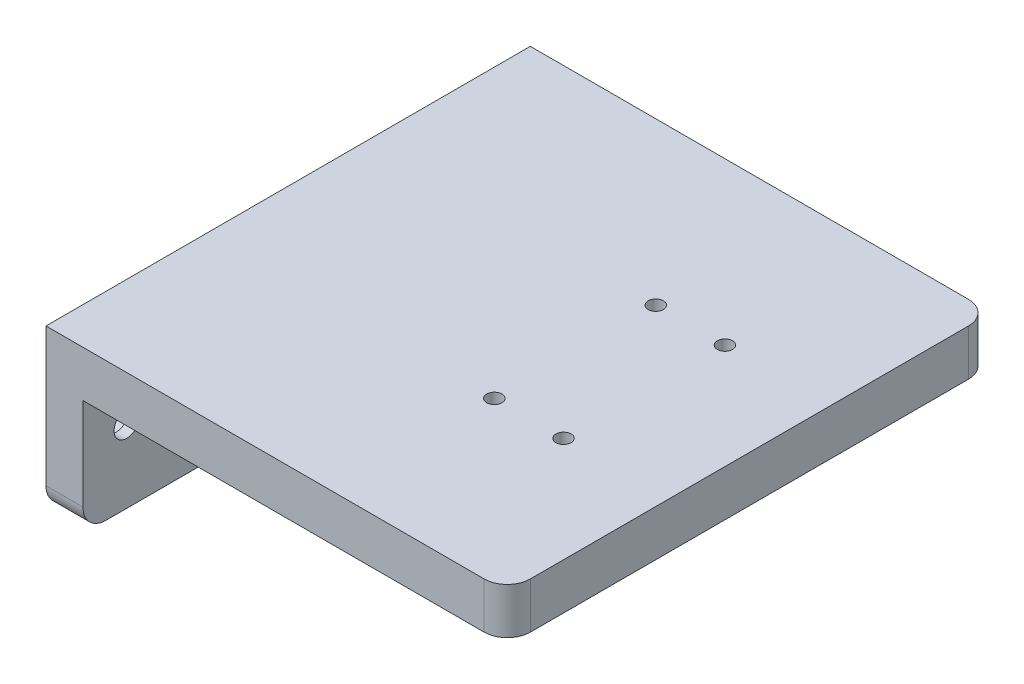
from build123d import *

# Parameters (mm, degrees)
EXTRUDE_1_DEPTH              = 27
SKETCH_2_R                   = 16
CUT_EXTRUDE_1_DEPTH          = 107.437775249
EXTRUDE_START                = -1.2
SKETCH_3_R                   = 16
SKETCH_3_R_2                 = 15
EXTRUDE_1_2_DEPTH            = 1.2
SKETCH_5_W                   = 100
SKETCH_5_H                   = 105
EXTRUDE_2_DEPTH              = 10
FILLET_1_R                   = 5
HOLE_WIZARD_M4_1_D           = 3.3
SKETCH_10_W                  = 21.869488537
SKETCH_10_H                  = 58.553791887
CUT_EXTRUDE_2_DEPTH          = 50
SKETCH_11_W                  = 105
SKETCH_11_H                  = 35
EXTRUDE_3_DEPTH              = 8
HOLE_WIZARD_M5_1_D           = 5.5
HOLE_WIZARD_M5_1_DEPTH       = 10.1
HOLE_WIZARD_M5_1_CBORE_D     = 10
HOLE_WIZARD_M5_1_CBORE_DEPTH = 5.7
HOLE_WIZARD_M5_1_TIP         = 1.652366702
FILLET_2_R                   = 5


with BuildPart() as part:
    # 草图1 → Extrude 1 (new, symmetric)
    with BuildSketch(Plane.XY):
        Polygon((90, 0), (0, 0), (0, 50), (-10, 50), (-10, -10), (90, -10), align=None)
    extrude(amount=EXTRUDE_1_DEPTH, both=True)

    # 草图2 → 切除-拉伸1 (cut, through all)
    with BuildSketch(Plane(origin=(0, 0, 0), x_dir=(0, 0, -1), z_dir=(1, 0, 0))):
        with Locations((0, 30)):
            Circle(SKETCH_2_R)
    extrude(amount=-CUT_EXTRUDE_1_DEPTH, mode=Mode.SUBTRACT)

    # 草图3 → Extrude 1 2 (add)
    with BuildSketch(Plane.ZY.offset(10).offset(EXTRUDE_START)):
        with Locations(Location((0, 30, 0), (0, 0, 180))):
            Circle(SKETCH_3_R)
        with Locations((0, 30)):
            Circle(SKETCH_3_R_2, mode=Mode.SUBTRACT)
    extrude(amount=EXTRUDE_1_2_DEPTH)

    # 草图5 → 凸台-拉伸2 (add)
    with BuildSketch(Plane(origin=(0, 0, 0), x_dir=(1, 0, 0), z_dir=(0, 1, 0))):
        with Locations((40, 0)):
            Rectangle(SKETCH_5_W, SKETCH_5_H)
    extrude(amount=-EXTRUDE_2_DEPTH)

    # 圆角1
    fillet_1_edges = [part.edges().sort_by_distance(p)[0] for p in [
        (-5, 50, 27),
        (90, -5, -52.5),
        (90, -5, 52.5),
        (-5, 50, -27),
    ]]
    fillet(fillet_1_edges, radius=FILLET_1_R)

    # M4 螺纹孔1 (through all)
    with Locations(Plane(origin=(67.2, 0, 17.5), x_dir=(0, 0, 1), z_dir=(0, 1, 0))):
        with Locations((0, 0), (0, -15), (-35, 0), (-35, -15)):
            Hole(HOLE_WIZARD_M4_1_D / 2)

    # 草图10 → 切除-拉伸2 (cut)
    with BuildSketch(Plane(origin=(0, 50, 0), x_dir=(1, 0, 0), z_dir=(0, 1, 0))):
        with Locations((-5.309523809, -0.493827161)):
            Rectangle(SKETCH_10_W, SKETCH_10_H)
    extrude(amount=-CUT_EXTRUDE_2_DEPTH, mode=Mode.SUBTRACT)

    # 草图11 → 凸台-拉伸3 (add)
    with BuildSketch(Plane.ZY.offset(10)):
        with Locations((0, -17.5)):
            Rectangle(SKETCH_11_W, SKETCH_11_H)
    extrude(amount=-EXTRUDE_3_DEPTH)

    # M5 六角圆柱头螺钉的柱形沉头孔1
    with Locations(Plane(origin=(-10, -19.1, -43), x_dir=(0, 0, -1), z_dir=(-1, 0, 0))):
        with Locations((0, 0), (-32, 0), (-54, 0), (-86, 0)):
            CounterBoreHole(HOLE_WIZARD_M5_1_D / 2, HOLE_WIZARD_M5_1_CBORE_D / 2, HOLE_WIZARD_M5_1_CBORE_DEPTH, depth=HOLE_WIZARD_M5_1_DEPTH)
            with Locations((0, 0, -(HOLE_WIZARD_M5_1_DEPTH + HOLE_WIZARD_M5_1_TIP / 2))):  # 118° drill point
                Cone(0, HOLE_WIZARD_M5_1_D / 2, HOLE_WIZARD_M5_1_TIP, mode=Mode.SUBTRACT)

    # 圆角2
    fillet_2_edges = [part.edges().sort_by_distance(p)[0] for p in [
        (-6, -35, -52.5),
        (-6, -35, 52.5),
    ]]
    fillet(fillet_2_edges, radius=FILLET_2_R)


solid = part.part
